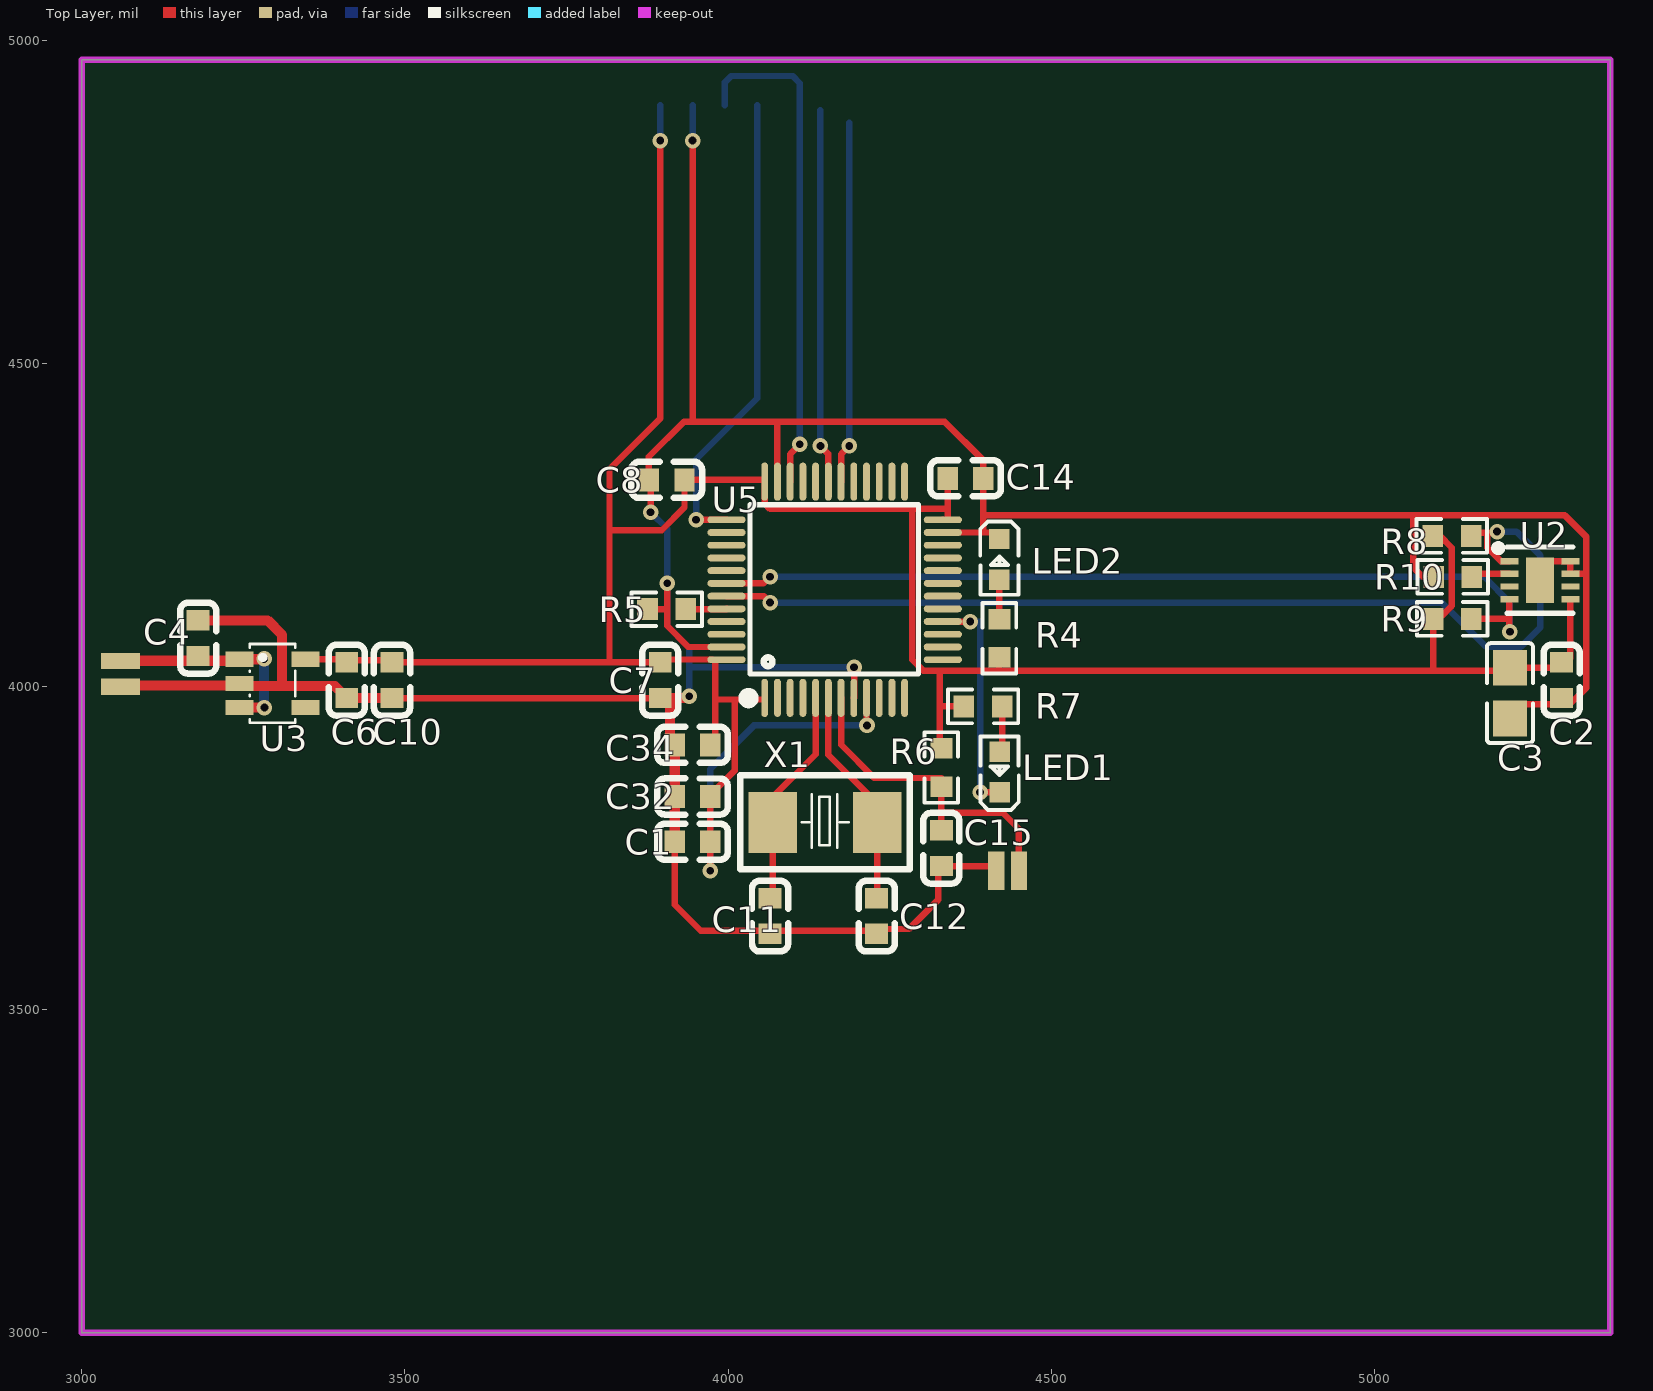
[diagram p0: Top Layer view]
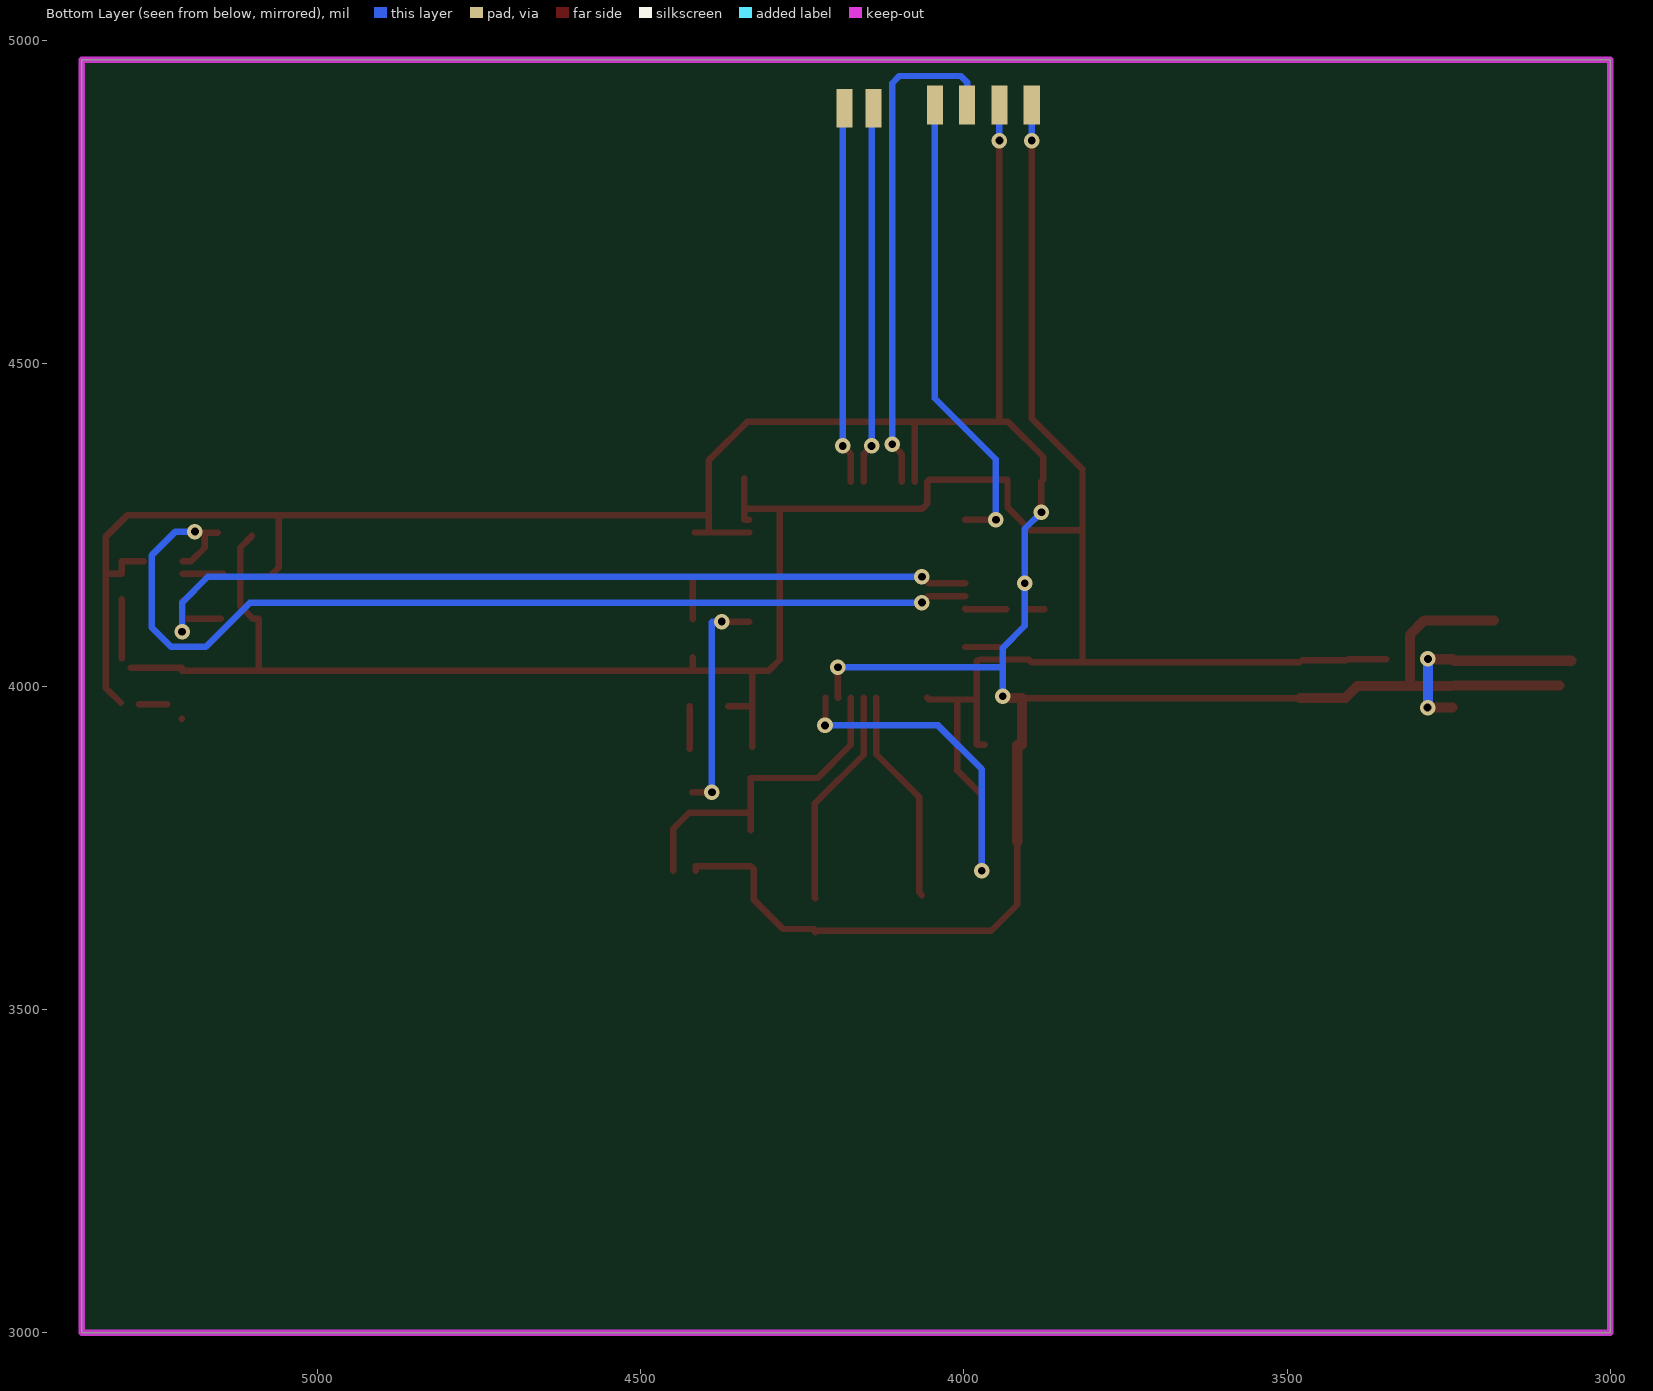
[diagram p1: Bottom Layer view, seen from below]
# Altium PCB MISC80717.pcbdoc
Units mil, origin at the board's own origin, x right, y up, seen from the top; angles counter-clockwise.
Board outline 2365 x 1970 mil, 2 copper layers (Top Layer, Bottom Layer), stack 1.928 mil thick; 27 components, 17 nets, 120 pads, 20 vias.

## Layer stack, top to bottom
Top Solder Mask Layer: solder mask 1.063, Dk 3.3
Top Layer: signal copper 0.472
Dielectric1: surface 0.984, FR4, Dk 4.5
Bottom Layer: signal copper 0.472
Bottom Solder Mask Layer: solder mask 1.063, Dk 3.3

## Board outline
3000,4970 3000,3000 5365,3000 5365,4970

## Design rules (kind name [scope] priority, off if disabled: settings)
BoardOutlineClearance copperThickness1oz [All] p0: genericclearance=10 ignorepadtopadclearanceinfootprint=FALSE except(0: Arc-SplitContinuation Track-SplitContinuation SMDPad-SplitContinuation THPad-SplitContinuation Via-SplitContinuation Fill-SplitContinuation Poly-SplitContinuation Region-SplitContinuation Text-SplitContinuation)
BoardOutlineClearance copperThickness2oz [All] p0: genericclearance=10 ignorepadtopadclearanceinfootprint=FALSE except(0: Arc-SplitContinuation Track-SplitContinuation SMDPad-SplitContinuation THPad-SplitContinuation Via-SplitContinuation Fill-SplitContinuation Poly-SplitContinuation Region-SplitContinuation Text-SplitContinuation)
BoardOutlineClearance otherClearance [All] p0: genericclearance=10 ignorepadtopadclearanceinfootprint=FALSE except(0: Arc-SplitContinuation Track-SplitContinuation SMDPad-SplitContinuation THPad-SplitContinuation Via-SplitContinuation Fill-SplitContinuation Poly-SplitContinuation Region-SplitContinuation Text-SplitContinuation)
Clearance copperThickness1oz [All] p1: gap=7 ignorepadtopadclearanceinfootprint=FALSE
Clearance copperThickness2oz [All] p1: gap=7 ignorepadtopadclearanceinfootprint=FALSE
Clearance otherClearance [All] p1: gap=7 ignorepadtopadclearanceinfootprint=FALSE
DiffPairsRouting differentialPair [All] p1: maxuncoupledlength=10 minlimit=6 maxlimit=Infinity mostfreqgap=6 toplayer_minwidth=5 toplayer_prefwidth=10 toplayer_maxwidth=100 bottomlayer_minwidth=5 bottomlayer_prefwidth=10 bottomlayer_maxwidth=100
PasteMaskExpansion pasteMaskExpansion [All] p1: expansion=0
PlaneConnect innerPlane [All] p1: planeconnectstyle=Relief reliefexpansion=20 reliefentries=4 reliefconductorwidth=10 reliefairgap=10
PolygonConnect copperRegion [All] p1: connectstyle=Relief reliefentries=4 reliefconductorwidth=10 polygonreliefangle="90 Angle" airgapwidth=10
RoutingVias viaSize [All] p1: viastyle="Through Hole" holewidth=12.0078 minholewidth=11.811 maxholewidth=248.0314 width=12.0078 minwidth=11.811 maxwidth=248.0314
SolderMaskExpansion solderMaskExpansion [IsVia] p1: useseparateexpansions=TRUE expansion=-1000 expansionbottom=-1000
SolderMaskExpansion solderMaskExpansion [All] p2: useseparateexpansions=TRUE expansion=2 expansionbottom=2
Width copperThickness1oz [All] p1: maxlimit=100 minlimit=5 preferedwidth=10
Width copperThickness2oz [All] p1: maxlimit=100 minlimit=8 preferedwidth=10

## Components (designator, comment, footprint, x,y, rotation, side; value= is the part's Value field where it differs from the comment)
C1 "1uF" C0603 3945,3760 r0 top
C2 "100nF" C0603 5290,4010 r270 top
C3 "4.7uF" C0805 5210,3990 r90 top
C4 "10uF" C0603 3180,4075 r270 top
C6 "10uF" C0603 3410,4010 r270 top
C7 "100nF" C0603 3895,4010 r90 top
C8 "100nF" C0603 3905,4320 r180 top
C10 "100nF" C0603 3480,4010 r90 top
C11 "20pF" C0603 4065,3645 r90 top
C12 "20pF" C0603 4230,3645 r90 top
C14 "100nF" C0603 4367.56,4322.44 r0 top
C15 "100nF" C0603 4330,3750 r270 top
C32 "100nF" C0603 3945,3830 r0 top
C34 "100nF" C0603 3945,3910 r180 top
LED1 "" LED_0603 4420,3870 r90 top
LED2 "" LED_0603 4420,4195 r270 top
R4 "1K" R0603 4420,4075 r90 top
R5 "10K" R0603 3905,4120 r180 top
R6 "10K" R0603 4330,3875 r90 top
R7 "1K" R0603 4394.59,3969.39 r0 top
R8 "10K" R0603 5120.14,4233.25 r180 top
R9 "10K" R0603 5120.66,4104.83 r180 top
R10 "10K" R0603 5121.34,4169.83 r180 top
U2 "SHT30-DIS-B2.5KS" DFN-8_L2.5-W2.5-P0.50-BL-EP 5256.34,4164.83 r270 top
U3 "TLV75533PDBVR" SOT-23-5_L3.0-W1.7-P0.95-LS2.8-BR 3295,4005 r180 top
U5 "STM32F103C8T6" LQFP-48_L7.0-W7.0-P0.50-LS9.0-BL 4165,4150 r0 top
X1 "8MHz" CRYSTAL-SMD_L5.0-W3.2 4150,3790 r180 top

## Footprints (in the part's own frame and the unit in brackets; to place one, negate y for a bottom-side part, rotate by r counter-clockwise, add the part's x,y. Pads: shape width x height; smd on the part's side, far side on the other; paste and mask are expansions set on the pad)
C0603 [mm]
  rect 0.8x0.9 smd: 1(-0.7,0) 2(0.7,0)
  silkscreen extent -1.39,-0.71 1.39,0.71
C0805 [mm]
  rect 1.41x1.35 smd paste-100 mask+0.051: 1(-1,0) 2(1,0)
  silkscreen extent -1.96,-0.9 1.96,0.9
CRYSTAL-SMD_L5.0-W3.2 [mm]
  rect 1.9x2.4 smd: 1(-2.05,0) 2(2.05,0)
  silkscreen extent -3.32,-1.85 3.33,1.85
DFN-8_L2.5-W2.5-P0.50-BL-EP [mm]
  rect 0.25x0.7 smd: 1(-0.75,-1.2) 2(-0.25,-1.2) 3(0.25,-1.2) 4(0.75,-1.2) 5(0.75,1.2) 6(0.25,1.2) 7(-0.25,1.2) 8(-0.75,1.2)
  rect 1.8x1.1 smd: 9(0,0)
  silkscreen extent -1.39,-1.77 1.3,1.3
LED_0603 [mil]
  rect 31.5x31.5 smd paste+0 mask+2: 1(-33.5,-0.4) 2(29.5,-0.2)
  silkscreen extent -61,-30 53,30
LQFP-48_L7.0-W7.0-P0.50-LS9.0-BL [mm]
  oval 0.27x1.5 smd paste+0 mask+0.05: 1(-2.75,-4.25) 2(-2.25,-4.25) 3(-1.75,-4.25) 4(-1.25,-4.25) 5(-0.75,-4.25) 6(-0.25,-4.25) 7(0.25,-4.25) 8(0.75,-4.25) 9(1.25,-4.25) 10(1.75,-4.25) 11(2.25,-4.25) 12(2.75,-4.25) 25(2.75,4.25) 26(2.25,4.25) 27(1.75,4.25) 28(1.25,4.25) 29(0.75,4.25) 30(0.25,4.25) 31(-0.25,4.25) 32(-0.75,4.25) 33(-1.25,4.25) 34(-1.75,4.25) 35(-2.25,4.25) 36(-2.75,4.25)
  oval 1.5x0.27 smd paste+0 mask+0.05: 13(4.25,-2.75) 14(4.25,-2.25) 15(4.25,-1.75) 16(4.25,-1.25) 17(4.25,-0.75) 18(4.25,-0.25) 19(4.25,0.25) 20(4.25,0.75) 21(4.25,1.25) 22(4.25,1.75) 23(4.25,2.25) 24(4.25,2.75) 37(-4.25,2.75) 38(-4.25,2.25) 39(-4.25,1.75) 40(-4.25,1.25) 41(-4.25,0.75) 42(-4.25,0.25) 43(-4.25,-0.25) 44(-4.25,-0.75) 45(-4.25,-1.25) 46(-4.25,-1.75) 47(-4.25,-2.25) 48(-4.25,-2.75)
  silkscreen extent -3.59,-4.46 3.3,3.34
R0603 [mil]
  rect 31.75x34.02 smd paste-3937.01 mask+2: 1(-29.66,0) 2(29.66,0)
  silkscreen extent -55,-26 55,26
SOT-23-5_L3.0-W1.7-P0.95-LS2.8-BR [mm]
  rect 1.1x0.6 smd: 1(1.3,-0.95) 2(1.3,0) 3(1.3,0.95) 4(-1.3,0.95) 5(-1.3,-0.95)
  silkscreen extent -0.9,-1.55 0.9,1.55

## Free pads (board coordinates)
  rect 25x60 smd far side: 1(4045,4900) 1(4140,4895) 2(3995,4900) 2(4185,4895) 3(3945,4900) 4(3895,4900)
  rect 25x60 smd: 1(4415,3715) 1(4450,3715)
  rect 60x25 smd: 3(3060,4000) 4(3060,4040)

## Via types
v1: diameter 24.02, hole 12, Top Layer to Bottom Layer, 20 vias

## Nets (pads, with @x,y where several pads share a name; then routed paths per layer and width w, separated by ;. In a path a pad name is that pad's centre, name@x,y a point inside that pad or via, vN(x,y) a via of type N, cw(c..) or ccw(c..) an arc to the next point about the centre after c; other vN are vias at no path point)
$1N55: R5.1 U5.44 | length 63.2
  Top Layer w10: R5.1 3997.21,4120 U5.44
$1N76: LED2.2 R4.2 | length 60.9
  Top Layer w10: LED2.2 4420,4165.3 R4.2
$1N102: LED1.2 R7.2 | length 65.8
  Top Layer w10: LED1.2@4424.25,3903.55 R7.2
$1N108: R10.1 U2.2 | length 63.2
  Top Layer w10: R10.1@5145.85,4174.68 U2.2
+3.3V: C1.2 C2.1 C3.2 C6.1 C7.2 C8.1 C10.2 C14.1 C32.2 C34.1 pad.4@3895,4900 R4.1 R6.2 R7.1 R8.2 R9.2 U2.5 U3.5 U5.1 U5.9 U5.24 U5.36 U5.48 | length 4929.8
  Top Layer w10: U3.5 C6.1@3405.16,4042.4 ; C6.1@3409.07,4040.75 C10.2@3476.81,4040.75 ; C10.2 3816.53,4037.56 ; v1(3895,4845) 3895,4415 3816.53,4336.53 3816.53,4242.28 ; C34.1@3967.56,3910 3979.51,3910 3980,3910.49 3980,3980 ; v1(3972.56,3715) C1.2 3972.56,3832.44 4010,3869.88 4010,3977.61 4007.46,3980.15 ; U5.48@3975.35,4042.07 3899.51,4042.07 C7.2 3816.53,4037.56 ; U5.48@3979.85,4039.85 3979.85,3980.15 4007.46,3980.15 ; U5.1 4054.2,3980.15 4007.46,3980.15 ; U5.9 4214.21,3940.79 v1(4215,3940) ; R6.2@4327.56,3907.1 4327.56,4022.62 ; 4328.87,3969.39 R7.1 ; U5.24 4340,4258.27 4340,4275.43 ; C14.1 4340,4275.43 ; R4.1 4420,4025.87 4419.13,4025 ; R8.2@5101.75,4233.25 5120,4215 5120,4125 5099.83,4104.83 R9.2 5091,4025.52 5091.52,4025 ; C2.1@5289.5,4029.5 5210.13,4029.5 C3.2 5210,4025 5091.52,4025 ; C2.1@5303.58,4043.58 U2.5 ; 3816.53,4037.56 3816.53,4242.28 ; 3816.53,4242.28 3897.28,4242.28 3932.56,4277.56 C8.1 4054.05,4320 U5.36 4056.73,4283.27 4065,4275 4282.41,4275 ; 4282.41,4275 4339.57,4275 4340,4275.43 ; 4282.41,4275 4285,4272.41 4285,4041.79 4301.79,4025 4419.13,4025 ; 4419.13,4025 5091.52,4025
  Bottom Layer w10: v1(3895,4845) pad.4@3895,4900 ; v1(3972.56,3715) 3972.56,3872.56 4040,3940 v1(4215,3940)
GND: C1.1 C2.2 C3.1 C4.1 C6.2 C7.1 C8.2 C10.1 C11.1 C12.1 C14.2 C15.2 C32.1 C34.2 LED2.1 pad.1@4415,3715 pad.3 R5.2 R10.2 U2.7 U2.8 U2.9 U3.2 U5.8 U5.23 U5.35 U5.47 | length 5691.3
  Top Layer w10: C10.1 C7.1 C7.1@3910,3982.44 ; R5.2 3900.67,4120 ; v1(3880,4270) 3880,4317.44 C8.2 3877.44,4355.63 3931.81,4410 3945.95,4410 ; v1(3905.79,4160) 3905.79,4094.21 3938.58,4061.42 U5.47 ; C1.1 3917.44,3662.56 3957.56,3622.44 4227.56,3622.44 C12.1@4230,3620 ; v1(3945,4845) 3945,4410.95 3945.95,4410 ; 4075,4410 3945.95,4410 ; U5.35 4076.42,4408.58 ; 4076.42,4410 4335,4410 4395.12,4349.88 C14.2 4395.12,4263.97 ; U5.8 4195,3983.15 v1(4195,4030) ; C12.1@4230,3622.44 4232.56,3625 4280,3625 4325,3670 4325,3717.44 C15.2 4415,3722.44 pad.1@4415,3715 ; U5.23 4393.68,4238.58 ; LED2.1@4416.42,4238.58 4393.68,4238.58 ; R10.2@5089.19,4170 5075,4170 5060,4185 5060,4265 ; C3.1 C3.1@5210.63,3950.63 ; C3.1@5233.01,3973.01 C2.2@5276.99,3973.01 ; U2.9@5269.36,4194.36 U2.8 U2.7 5327.75,4174.68 5328.35,4174.08 ; C2.2@5305,3975 5328.35,3998.35 5328.35,4174.08 ; 4393.68,4238.58 4395.12,4240.02 4395.12,4263.97 ; 4395.12,4263.97 4396.15,4265 5060,4265 ; 5060,4265 5295,4265 5328.35,4231.65 5328.35,4174.08
  Top Layer w15.75: pad.3@3078.15,4001.85 U3.2@3240.67,4001.85 ; C4.1 3287.44,4102.56 3309.94,4080.06 3309.94,4000.99 ; U3.2@3247.82,4000.99 3309.94,4000.99 ; C10.1 C6.2 3391.45,4000.99 3309.94,4000.99 ; C1.1 C32.1 C34.2 3910,3910 3910,3982.44 3937.44,3982.44 v1(3940,3985)
  Bottom Layer w10: v1(3880,4270) 3905.79,4244.21 v1(3905.79,4160) 3905.79,4094.21 3940,4060 3940,4028.47 ; v1(3940,3985) 3940,4028.47 ; v1(3945,4845) pad.3@3945,4900 ; v1(4195,4030) 3941.53,4030 3940,4028.47
OSCIN: C11.2 U5.5 X1.2 | length 334.3
  Top Layer w10: C11.2@4065,3677.56 4069.29,3681.85 X1.2 4069.29,3829.29 4135.47,3895.47 U5.5
OSCOUT: C12.2 U5.6 X1.1 | length 341.7
  Top Layer w10: U5.6 4155.16,3894.84 4230.71,3819.29 X1.1 4230.71,3673.27 C12.2
PA6: LED1.1 U5.16 | length 350.8
  Top Layer w10: U5.16 v1(4374.81,4100.78) ; v1(4390,3836.5) LED1.1
  Bottom Layer w10: v1(4374.81,4100.78) 4389.22,4100.78 ; v1(4390,3836.5) 4390,4100
PA9: pad.2@4185,4895 U5.30 | length 560.4
  Top Layer w10: U5.30 4175,4317.48 4175,4360 v1(4187.5,4372.5)
  Bottom Layer w10: v1(4187.5,4372.5) pad.2@4187.5,4872.5
PA10: pad.1@4140,4895 U5.31 | length 579.9
  Top Layer w10: v1(4142.87,4372.5) 4155.16,4360.21 U5.31
  Bottom Layer w10: v1(4142.87,4372.5) pad.1@4142.87,4892.13
PB6: R9.1 U2.4 U5.42 | length 1384.8
  Top Layer w10: U5.42 4054.84,4159.84 v1(4065,4170) ; R9.1 5208.56,4104.83 ; U2.4@5209.09,4133.09 5209.09,4085.91 v1(5210,4085)
  Bottom Layer w10: v1(4065,4170) 5170,4170 5210,4130 v1(5210,4085)
PB7: R8.1 U2.1 U5.43 | length 1598.5
  Top Layer w10: U5.43 4055,4140.16 v1(4065.08,4130.08) ; R8.1@5154.8,4238.25 5188.25,4238.25 v1(5190,4240) ; 5175,4237.47 5175,4215 5195.64,4194.36 U2.1
  Bottom Layer w10: v1(4065.08,4130.08) 5104.92,4130.08 5172.99,4062.01 5227.01,4062.01 5257.07,4092.07 5257.07,4202.93 5220,4240 v1(5190,4240)
RST: C15.1 pad.1@4450,3715 R6.1 U5.7 | length 525.5
  Top Layer w10: U5.7 4175,3982.52 4175,3910 4226.3,3858.7 4330,3858.7 R6.1 4330,3805 ; C15.1 4330,3805 ; pad.1@4450,3715 4450,3780 4425,3805 4330,3805
SWCLK: pad.1@4045,4900 U5.37 | length 728
  Top Layer w10: v1(3950.55,4258.27) U5.37
  Bottom Layer w10: v1(3950.55,4258.27) 3950.55,4351.94 4045,4446.39 pad.1@4045,4900
SWDIO: pad.2@3995,4900 U5.34 | length 782.6
  Top Layer w10: U5.34 4096.1,4360 v1(4111.1,4375)
  Bottom Layer w10: pad.2@3995,4900 3995,4935 4005,4945 4100,4945 4111.1,4933.9 v1(4111.1,4375)
VIN: C4.2 pad.4@3060,4040 U3.1 U3.3 | length 334.1
  Top Layer w15.75: pad.4@3060,4040 U3.1@3241.41,4040 ; U3.3 v1(3282.55,3967.6) ; U3.1 3281.46,4042.4 v1(3282.01,4042.95)
  Bottom Layer w15.75: v1(3282.01,4042.95) 3282.01,3968.14 v1(3282.55,3967.6)
pads on no net: U2.3 U2.6 U3.4 U5.2 U5.3 U5.4 U5.10 U5.11 U5.12 U5.13 U5.14 U5.15 U5.17 U5.18 U5.19 U5.20 U5.21 U5.22 U5.25 U5.26 U5.27 U5.28 U5.29 U5.32 U5.33 U5.38 U5.39 U5.40 U5.41 U5.45 U5.46

## Keep-outs
Board Outline Layer:
  the board outline again, w10

## Silkscreen, mask and mechanical layers (free items; w line width, h text height)
Top Stiffener Layer:
  region: 3000,4970 3000,3000 5365,3000 5365,4970
Bottom Stiffener Layer:
  region: 3000,4970 3000,3000 5365,3000 5365,4970
  region: 3000,4970 3000,3000 5365,3000 5365,4970

## Dimensions
3000,5395 to 5366.27,5395 on Document Layer
5995,4970 to 5995,3000 on Document Layer